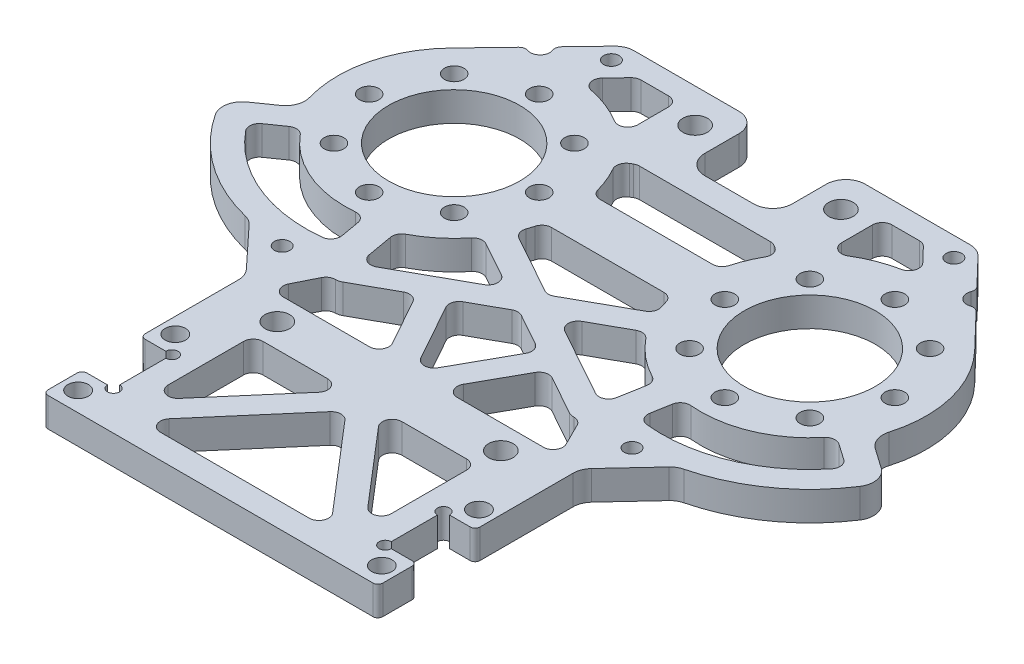
SolidWorks part; units mm, degrees
material "Thornel Mat VMA"
ref_plane "Front Plane" through (0, 0, 0) normal (0, 0, 1) x (1, 0, 0)
ref_plane "Top Plane" through (0, 0, 0) normal (0, 1, 0) x (1, 0, 0)
ref_plane "Right Plane" through (0, 0, 0) normal (1, 0, 0) x (0, 0, -1)
sketch "Sketch1" plane through (0, 0, 0) normal (0, 1, 0) x (1, 0, 0)
  line L0 (-15, 28) -> (15, 28) construction
  line L1 (-23, -50) -> (23, -50) construction
  line L2 (0, 28) -> (0, -50) construction
  line L3 (-36.6, 0) -> (36.6, 0) construction
  line L4 (-36.2611, 35) -> (-9, 35)
  line L5 (36.2611, 35) -> (53.9095, 16.6248)
  line L9 (-36.2611, 35) -> (-53.9095, 16.6248)
  line L11 (-34.45, -86.75) -> (34.45, -86.75)
  line L12 (34.45, -86.75) -> (34.45, -78.75)
  line L13 (-34.45, -66.75) -> (-29.2, -66.75)
  line L14 (-27.95, -68) -> (-27.95, -77.5)
  line L15 (-29.2, -78.75) -> (-34.45, -78.75)
  line L16 (-34.45, -78.75) -> (-34.45, -86.75)
  line L17 (27.95, -68) -> (27.95, -77.5)
  line L18 (34.45, -66.75) -> (29.2, -66.75)
  line L19 (29.2, -78.75) -> (34.45, -78.75)
  line L21 (-34.45, -66.75) -> (-34.45, -45)
  line L22 (34.45, -66.75) -> (34.45, -45)
  line L23 (-9, 35) -> (-9, 20)
  line L24 (9, 35) -> (9, 20)
  line L25 (-9, 20) -> (9, 20)
  line L26 (9, 35) -> (36.2611, 35)
  line L27 (-58.6962, -9.368) -> (-68.2579, -16.0632)
  line L28 (-55.0309, -12.9055) -> (-61.5841, -17.4941)
  line L29 (-32.6929, -22.1582) -> (-31.3037, -30.0366)
  line L30 (55.0309, -12.9055) -> (61.5841, -17.4941)
  line L31 (-36.6, 0) -> (-48.9744, -12.3744) construction
  line L32 (-36.6, 0) -> (-36.6, -17.5) construction
  line L33 (32.6929, -22.1582) -> (31.3037, -30.0366)
  line L34 (58.6962, -9.368) -> (68.2579, -16.0632)
  line L35 (-34.45, -45) -> (-44.0313, -34.7135)
  line L36 (34.45, -45) -> (44.0313, -34.7135)
  line L37 (36, -36) -> (-36, -36) construction
  circle A0 centre (-36.6, 0) radius 13.5
  circle A2 centre (-15, 28) radius 2.525
  circle A3 centre (15, 28) radius 2.525
  circle A4 centre (-23, -50) radius 2.525
  circle A5 centre (23, -50) radius 2.525
  circle A6 centre (-36.6, 0) radius 17.5 construction
  circle A7 centre (36.6, 0) radius 13.5
  circle A8 centre (36.6, 0) radius 17.5 construction
  circle A9 centre (-36.6, 17.5) radius 2.01
  circle A10 centre (-24.2256, 12.3744) radius 2.01
  circle A11 centre (-19.1, 0) radius 2.01
  circle A12 centre (-24.2256, -12.3744) radius 2.01
  circle A13 centre (-36.6, -17.5) radius 2.01
  circle A14 centre (-48.9744, -12.3744) radius 2.01
  circle A15 centre (-54.1, 0) radius 2.01
  circle A16 centre (-48.9744, 12.3744) radius 2.01
  circle A17 centre (48.9744, 12.3744) radius 2.01
  circle A18 centre (54.1, 0) radius 2.01
  circle A19 centre (48.9744, -12.3744) radius 2.01
  circle A20 centre (36.6, -17.5) radius 2.01
  circle A21 centre (24.2256, -12.3744) radius 2.01
  circle A22 centre (19.1, 0) radius 2.01
  circle A23 centre (24.2256, 12.3744) radius 2.01
  circle A24 centre (36.6, 17.5) radius 2.01
  arc A25 (-53.9095, 16.6248) -> (-58.6962, -9.368) centre (-36.6, 0) ccw
  arc A26 (53.9095, 16.6248) -> (58.6962, -9.368) centre (36.6, 0) cw
  arc A31 (-27.95, -68) -> (-29.2, -66.75) centre (-27.95, -66.75) ccw
  arc A32 (-29.2, -78.75) -> (-27.95, -77.5) centre (-27.95, -78.75) ccw
  arc A33 (29.2, -78.75) -> (27.95, -77.5) centre (27.95, -78.75) cw
  arc A34 (27.95, -68) -> (29.2, -66.75) centre (27.95, -66.75) cw
  circle A35 centre (-31.25, -82.75) radius 2.1
  circle A36 centre (-31.25, -62.75) radius 2.1
  circle A37 centre (31.25, -82.75) radius 2.1
  circle A38 centre (31.25, -62.75) radius 2.1
  circle A39 centre (-35.25, 31) radius 1.6
  circle A40 centre (35.25, 31) radius 1.6
  circle A42 centre (-15, 28) radius 7 construction
  circle A43 centre (15, 28) radius 7 construction
  arc A44 (-61.5841, -17.4941) -> (-31.3037, -30.0366) centre (-36.6, 0) ccw
  arc A45 (-68.2579, -16.0632) -> (-44.0313, -34.7135) centre (-36.6, 0) ccw
  arc A46 (-55.0309, -12.9055) -> (-32.6929, -22.1582) centre (-36.6, 0) ccw
  arc A47 (55.0309, -12.9055) -> (32.6929, -22.1582) centre (36.6, 0) cw
  arc A48 (61.5841, -17.4941) -> (31.3037, -30.0366) centre (36.6, 0) cw
  arc A49 (68.2579, -16.0632) -> (44.0313, -34.7135) centre (36.6, 0) cw
  circle A50 centre (-36, -36) radius 1.6
  circle A51 centre (36, -36) radius 1.6
  point P36 (-36.6, 0)
  dimension "D1" = 27
  dimension "D2" = 30
  dimension "D6" = 35
  dimension "D8" = 5.05
  dimension "D9" = 8
  dimension "D10" = 4.02
  dimension "D11" = 3.2
  dimension "D13" = 8
  dimension "D15" = 24
  dimension "D16" = 1.25
  dimension "D19" = 4.2
  dimension "D23" = 3.2
  dimension "D30" = 10
  dimension "D31" = 5
  dimension "D34" = 22.5
  dimension "D35" = 3.2
  dimension "D3" = 46
  dimension "D4" = 78
  dimension "D5" = 28
  dimension "D7" = 73.2
  dimension "D12" = 20
  dimension "D14" = 62.5
  dimension "D17" = 3.3
  dimension "D18" = 12
  dimension "D20" = 4
  dimension "D21" = 4
  dimension "D22" = 12.75
  dimension "D24" = 3
  dimension "D25" = 70.5
  dimension "D26" = 7
  dimension "D27" = 3.5
  dimension "D28" = 18
  dimension "D29" = 8
  dimension "D32" = 5
  dimension "D33" = 10
  dimension "D36" = 36
  dimension "D37" = 72
  dimension "D38" = 5
  dimension "D39" = 5
extrude "Boss-Extrude1" add sketch "Sketch1" along normal blind 6
sketch "Sketch3" plane through (0, 6, 0) normal (0, 1, 0) x (1, 0, 0)
  line L0 (0, 35) -> (0, -86.75) construction
  line L1 (-35.7483, 23.9849) -> (-29.4909, 30.5)
  line L2 (-34.45, -86.75) -> (34.45, -86.75) construction
  line L3 (-36.6, 0) -> (36.6, 0) construction
  line L4 (-13.1266, 5) -> (13.1266, 5)
  line L5 (-13.1266, -5) -> (13.1266, -5)
  line L6 (-16.7122, 13.4341) -> (-14, 15)
  line L7 (16.7122, 13.4341) -> (14, 15)
  line L8 (-14, 15) -> (14, 15)
  line L9 (-26.6559, -21.843) -> (-24.5123, -34)
  line L10 (26.6559, -21.843) -> (24.5123, -34)
  line L11 (-30, -45) -> (30, -45)
  line L12 (-15, 28) -> (15, 28) construction
  line L13 (-23, -50) -> (23, -50) construction
  line L14 (-27.95, -68) -> (-27.95, -77.5) construction
  line L15 (19.656, -81.75) -> (-19.656, -81.75)
  line L16 (22.95, -77.9106) -> (22.95, -55)
  line L17 (22.95, -55) -> (3.294, -55)
  line L18 (-22.95, -77.9106) -> (-22.95, -55)
  line L19 (22.95, -81.75) -> (-22.95, -55) construction
  line L20 (22.95, -55) -> (-22.95, -81.75) construction
  line L21 (-22.95, -81.75) -> (0, -55) construction
  line L22 (0, -55) -> (22.95, -81.75) construction
  line L23 (-3.294, -55) -> (-22.95, -77.9106)
  line L24 (0, -58.8394) -> (-19.656, -81.75)
  line L25 (0, -58.8394) -> (19.656, -81.75)
  line L26 (3.294, -55) -> (22.95, -77.9106)
  line L27 (-3.294, -55) -> (-22.95, -55)
  line L28 (-9, 35) -> (-36.2611, 35) construction
  line L29 (-24.5123, -34) -> (-30, -45)
  line L30 (24.5123, -34) -> (30, -45)
  line L31 (-31.3037, -30.0366) -> (-32.6929, -22.1582) construction
  line L32 (-24.5123, -34) -> (15.6273, -11.6682) construction
  line L33 (-25.7278, -31.8153) -> (14.4119, -9.4835)
  line L34 (-23.2969, -36.1847) -> (16.8428, -13.8529)
  line L35 (24.5123, -34) -> (-15.6273, -11.6682) construction
  line L36 (25.7278, -31.8153) -> (-14.4119, -9.4835)
  line L37 (23.2969, -36.1847) -> (-16.8428, -13.8529)
  line L38 (0, -50) -> (-12.5915, -27.3678) construction
  line L39 (-2.1847, -51.2154) -> (-14.7761, -28.5832)
  line L40 (2.1847, -48.7846) -> (-10.4068, -26.1524)
  line L41 (0, -50) -> (12.5915, -27.3678) construction
  line L42 (2.1847, -51.2154) -> (14.7761, -28.5832)
  line L43 (-2.1847, -48.7846) -> (10.4068, -26.1524)
  line L44 (-29.4909, 30.5) -> (-21, 30.5)
  line L45 (-21, 30.5) -> (-21, 18.2384)
  line L46 (-36.2611, 35) -> (-53.9095, 16.6248) construction
  line L47 (29.4909, 30.5) -> (21, 30.5)
  line L48 (35.7483, 23.9849) -> (29.4909, 30.5)
  line L49 (21, 30.5) -> (21, 18.2384)
  arc A0 (-13.1266, 5) -> (-16.7122, 13.4341) centre (-36.6, 0) ccw
  arc A1 (13.1266, 5) -> (16.7122, 13.4341) centre (36.6, 0) cw
  arc A2 (-53.9095, 16.6248) -> (-58.6962, -9.368) centre (-36.6, 0) ccw construction
  arc A3 (-26.6559, -21.843) -> (-13.1266, -5) centre (-36.6, 0) ccw
  arc A4 (26.6559, -21.843) -> (13.1266, -5) centre (36.6, 0) cw
  arc A5 (-25.7278, -31.8153) -> (-23.2969, -36.1847) centre (-24.5123, -34) ccw
  arc A6 (16.8428, -13.8529) -> (14.4119, -9.4835) centre (15.6273, -11.6682) ccw
  arc A7 (25.7278, -31.8153) -> (23.2969, -36.1847) centre (24.5123, -34) cw
  arc A8 (-16.8428, -13.8529) -> (-14.4119, -9.4835) centre (-15.6273, -11.6682) cw
  arc A9 (-2.1847, -51.2154) -> (2.1847, -48.7846) centre (0, -50) ccw
  arc A10 (-10.4068, -26.1524) -> (-14.7761, -28.5832) centre (-12.5915, -27.3678) ccw
  arc A11 (2.1847, -51.2154) -> (-2.1847, -48.7846) centre (0, -50) cw
  arc A12 (10.4068, -26.1524) -> (14.7761, -28.5832) centre (12.5915, -27.3678) cw
  arc A13 (-35.7483, 23.9849) -> (-21, 18.2384) centre (-36.6, 0) cw
  arc A14 (35.7483, 23.9849) -> (21, 18.2384) centre (36.6, 0) ccw
  point P35 (0, -68.375)
  point P51 (-4.4425, -22.8341)
  point P58 (4.4425, -22.8341)
  point P65 (-6.2957, -38.6839)
  point P72 (6.2957, -38.6839)
  dimension "D1" = 10
  dimension "D14" = 8
  dimension "D2" = 13
  dimension "D3" = 150
  dimension "D4" = 28
  dimension "D5" = 5
  dimension "D6" = 6
  dimension "D7" = 5
  dimension "D8" = 5
  dimension "D9" = 5
  dimension "D10" = 5
  dimension "D11" = 5
  dimension "D12" = 60
  dimension "D13" = 11
  dimension "D15" = 4.5
  dimension "D16" = 6
extrude "Cut-Extrude1" cut sketch "Sketch3" against normal through all contours L1 A13 L45 L44 | A14 L48 L47 L49 | L4 A1 L7 L8 L6 A0 | A3 A8 L36 L33 A6 A4 L5 | L37 A8 A3 L9 L33 | A5 L29 L11 L39 L34 | L40 L43 L37 L34 | A6 L34 L36 L10 A4 | L30 A7 L37 L42 L11 | L23 L27 L18 | L25 L24 L15 | L17 L26 L16
fillet "R2 cutout fillet" radius 2 56 edges at (-13.1266, 3, 5) (13.1266, 3, 5) (26.6559, 3, 21.843) (-26.6559, 3, 21.843) (22.95, 3, 55) (22.95, 3, 77.9106) (3.294, 3, 55) (19.656, 3, 81.75) (-19.656, 3, 81.75) (0, 3, 58.8394) (-3.294, 3, 55) (-22.95, 3, 77.9106) (-22.95, 3, 55) (-16.7122, 3, -13.4341) (14, 3, -15) (16.7122, 3, -13.4341) (13.1266, 3, -5) (-13.1266, 3, -5) (-14, 3, -15) (21, 3, -30.5) (29.4909, 3, -30.5) (35.7483, 3, -23.9849) (21, 3, -18.2384) (-5.1422, 3, 20.3625) (-24.9717, 3, 31.3947) (-16.9549, 3, 13.7866) (-14.5273, 3, 9.4232) (14.5273, 3, 9.4232) (16.9549, 3, 13.7866) (0, 3, 17.5016) (24.9717, 3, 31.3947) (5.1422, 3, 20.3625) (5.6426, 3, 45) (13.5607, 3, 30.7679) (25.6284, 3, 36.2371) (30, 3, 45) (-13.5607, 3, 30.7679) (-5.6426, 3, 45) (-30, 3, 45) (-25.6284, 3, 36.2371) (0, 3, 23.2234) (9.1914, 3, 28.337) (0, 3, 44.8578) (-9.1914, 3, 28.337) (-21, 3, -30.5) (-21, 3, -18.2384) (-35.7483, 3, -23.9849) (61.5841, 3, 17.4941) (31.3037, 3, 30.0366) (32.6929, 3, 22.1582) (55.0309, 3, 12.9055) (-31.3037, 3, 30.0366) (-61.5841, 3, 17.4941) (-55.0309, 3, 12.9055) (-32.6929, 3, 22.1582) (-29.4909, 3, -30.5)
fillet "R1 plug-in fillet" radius 1 6 edges at (34.45, 3, 66.75) (34.45, 3, 78.75) (34.45, 3, 86.75) (-34.45, 3, 86.75) (-34.45, 3, 78.75) (-34.45, 3, 66.75)
fillet "R4 outer edge fillet" radius 4 14 edges at (34.45, 3, 45) (44.0313, 3, 34.7135) (68.2579, 3, 16.0632) (58.6962, 3, 9.368) (-34.45, 3, 45) (-44.0313, 3, 34.7135) (-68.2579, 3, 16.0632) (-58.6962, 3, 9.368) (36.2611, 3, -35) (9, 3, -35) (9, 3, -20) (-9, 3, -20) (-9, 3, -35) (-36.2611, 3, -35)
sketch "Sketch4" plane through (0, 6, 0) normal (0, 1, 0) x (1, 0, 0)
  line L0 (-37.4416, 33.7708) -> (-53.9095, 16.6248) construction
  line L1 (-42.7146, 28.2807) -> (-47.0956, 23.7193)
  line L2 (0, 20) -> (0, 0) construction
  line L3 (5, 20) -> (-5, 20) construction
  line L4 (42.7146, 28.2807) -> (47.0956, 23.7193)
  arc A0 (-45.5386, 24.103) -> (-43.0351, 26.7095) centre (-44.9051, 26) ccw
  arc A1 (-45.5386, 24.103) -> (-47.0956, 23.7193) centre (-46.0137, 22.6802) ccw
  arc A2 (-42.7146, 28.2807) -> (-43.0351, 26.7095) centre (-41.6327, 27.2417) ccw
  arc A3 (45.5386, 24.103) -> (47.0956, 23.7193) centre (46.0137, 22.6802) cw
  arc A4 (42.7146, 28.2807) -> (43.0351, 26.7095) centre (41.6327, 27.2417) cw
  arc A5 (45.5386, 24.103) -> (43.0351, 26.7095) centre (44.9051, 26) cw
  dimension "D1" = 2
  dimension "D2" = 1.5
  dimension "D3" = 26
extrude "73.20 marking" cut sketch "Sketch4" against normal through all
